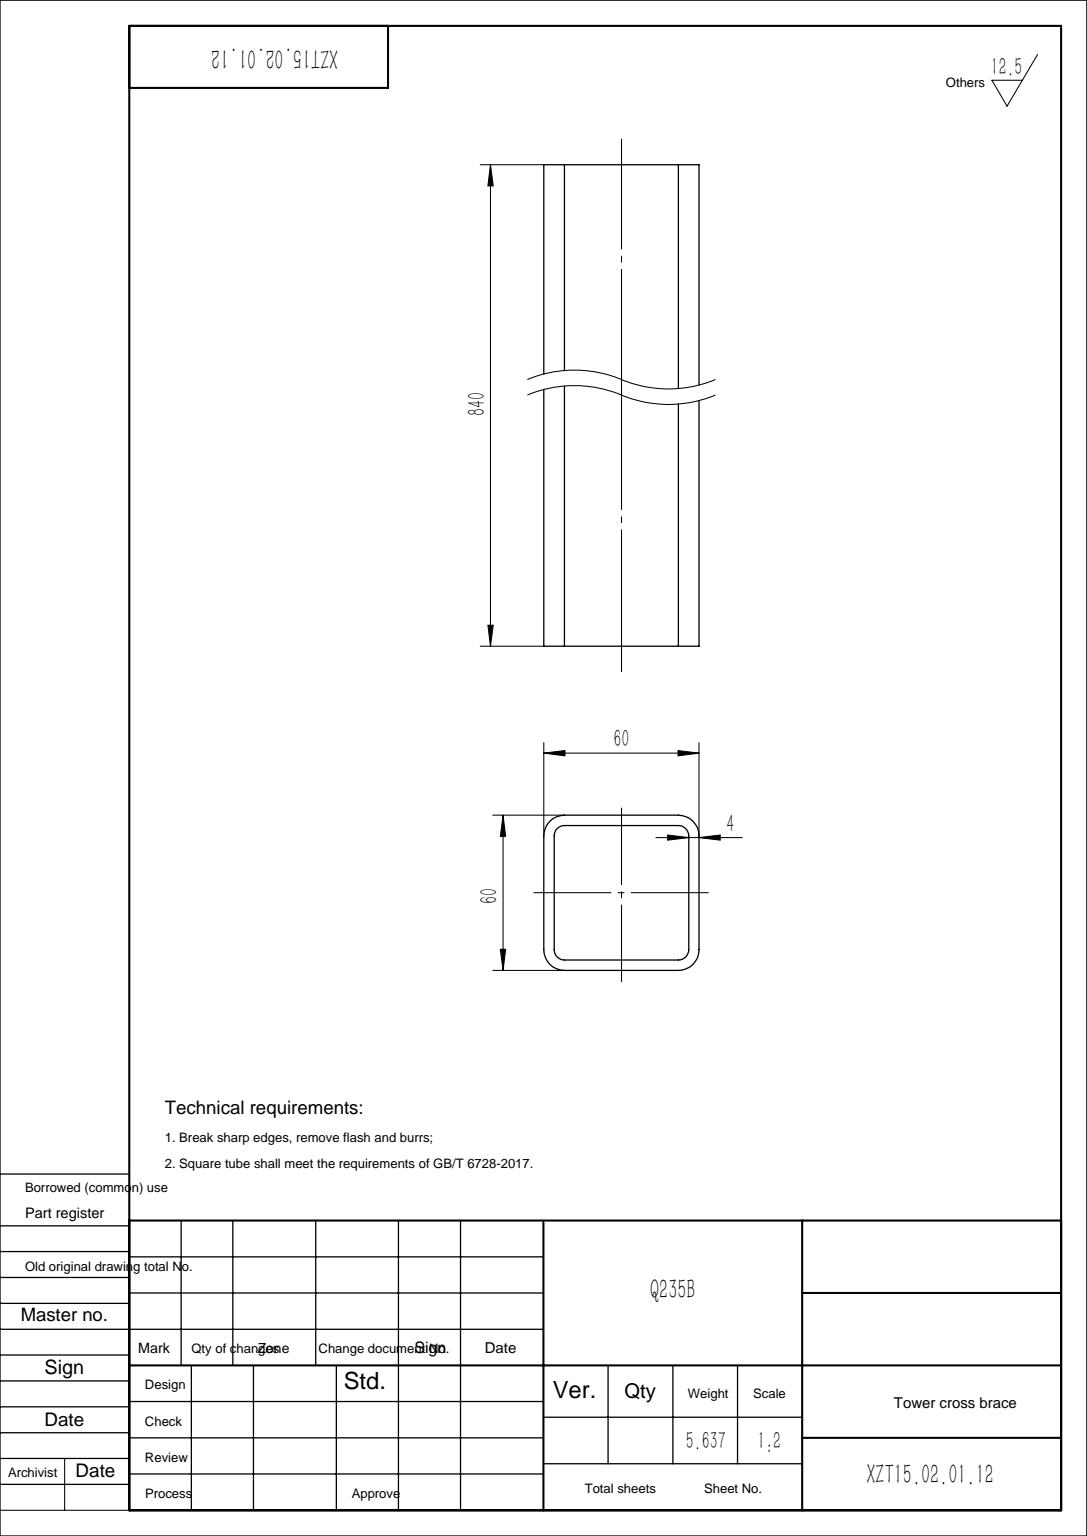
SolidWorks part; units mm, degrees
material "Q235B"
ref_plane "Front Plane" through (0, 0, 0) normal (0, 0, 1) x (1, 0, 0)
ref_plane "Top Plane" through (0, 0, 0) normal (0, 1, 0) x (1, 0, 0)
ref_plane "Right Plane" through (0, 0, 0) normal (1, 0, 0) x (0, 0, -1)
sketch "草图1" plane through (0, 0, 0) normal (0, 0, 1) x (1, 0, 0)
  line L0 (0, 0) -> (0, 840)
  dimension "D1" = 840
other "GB/T 6728-2002 square hollow section 60×60×4(1)"
ref_plane "Plane1" through (0, 0, 0) normal (0, 1, 0) x (-1, 0, 0)
sketch "Sketch1" plane through (0, 0, 0) normal (0, 1, 0) x (-1, 0, 0)
  line L0 (-22, -26) -> (22, -26)
  line L1 (-26, -22) -> (-26, 22)
  line L2 (22, 26) -> (-22, 26)
  line L3 (26, 22) -> (26, -22)
  line L4 (-22, -30) -> (22, -30)
  line L5 (-30, -22) -> (-30, 22)
  line L6 (22, 30) -> (-22, 30)
  line L7 (30, 22) -> (30, -22)
  arc A0 (30, 22) -> (22, 30) centre (22, 22) ccw
  arc A1 (22, -30) -> (30, -22) centre (22, -22) ccw
  arc A2 (-30, -22) -> (-22, -30) centre (-22, -22) ccw
  arc A3 (-22, 30) -> (-30, 22) centre (-22, 22) ccw
  arc A4 (-22, 26) -> (-26, 22) centre (-22, 22) ccw
  arc A5 (26, 22) -> (22, 26) centre (22, 22) ccw
  arc A6 (22, -26) -> (26, -22) centre (22, -22) ccw
  arc A7 (-26, -22) -> (-22, -26) centre (-22, -22) ccw
  point P0 (-30, 0)
  point P1 (30, 0)
  point P2 (0, 30)
  point P3 (0, -30)
  point P4 (0, 0)
  point P5 (-30, -30)
  point P6 (30, -30)
  point P7 (30, 30)
  point P8 (-30, 30)
  point P33 (0, 0)
  dimension "D1" = 8
  dimension "Thickness" = 4
  dimension "V_leg" = 60
